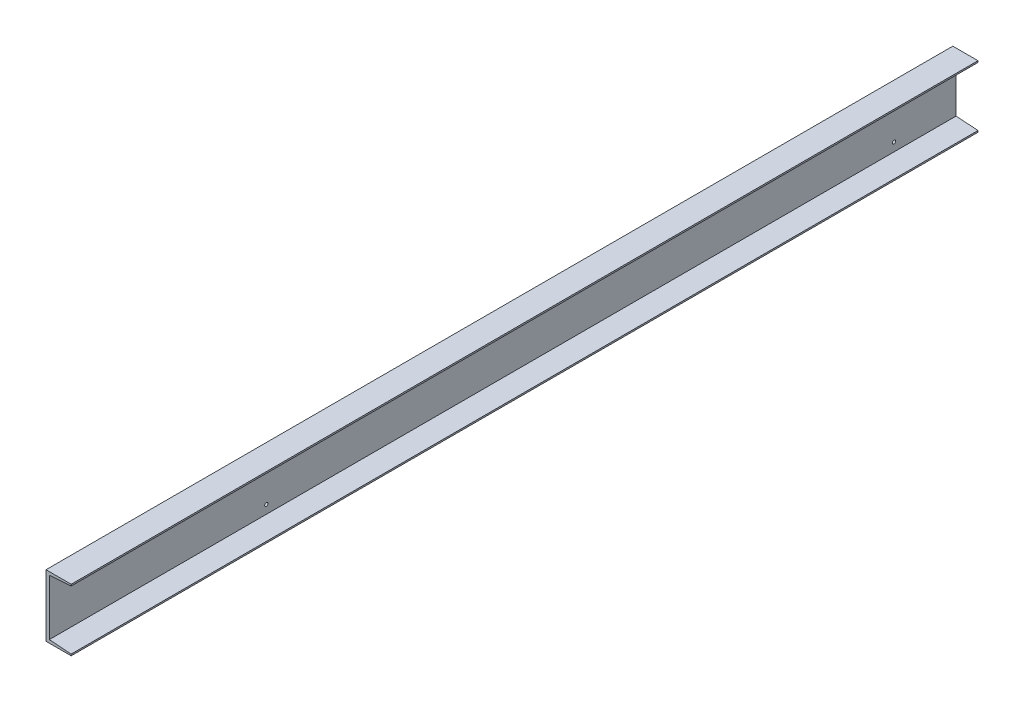
from build123d import *

# Parameters (mm, degrees)
EXTRUDE_1_DEPTH         = 1170
HOLE_WIZARD_M10_1_D     = 8.5
HOLE_WIZARD_M10_1_DEPTH = 27.5
HOLE_WIZARD_M10_1_TIP   = 2.553657631


with BuildPart() as part:
    # 草图1 → 凸台-拉伸1 (new, symmetric)
    with BuildSketch(Plane.XY):
        Polygon((0, 0), (65, 0), (65, 4), (8.5, 8), (8.5, 152), (65, 156), (65, 160), (0, 160), align=None)
    extrude(amount=EXTRUDE_1_DEPTH, both=True)

    # M10 螺纹孔1
    with Locations(Plane.ZY):
        with Locations((-1010, 30), (610, 30), (-1010, 130), (610, 130)):
            Hole(HOLE_WIZARD_M10_1_D / 2, depth=HOLE_WIZARD_M10_1_DEPTH)
            with Locations((0, 0, -(HOLE_WIZARD_M10_1_DEPTH + HOLE_WIZARD_M10_1_TIP / 2))):  # 118° drill point
                Cone(0, HOLE_WIZARD_M10_1_D / 2, HOLE_WIZARD_M10_1_TIP, mode=Mode.SUBTRACT)


solid = part.part
